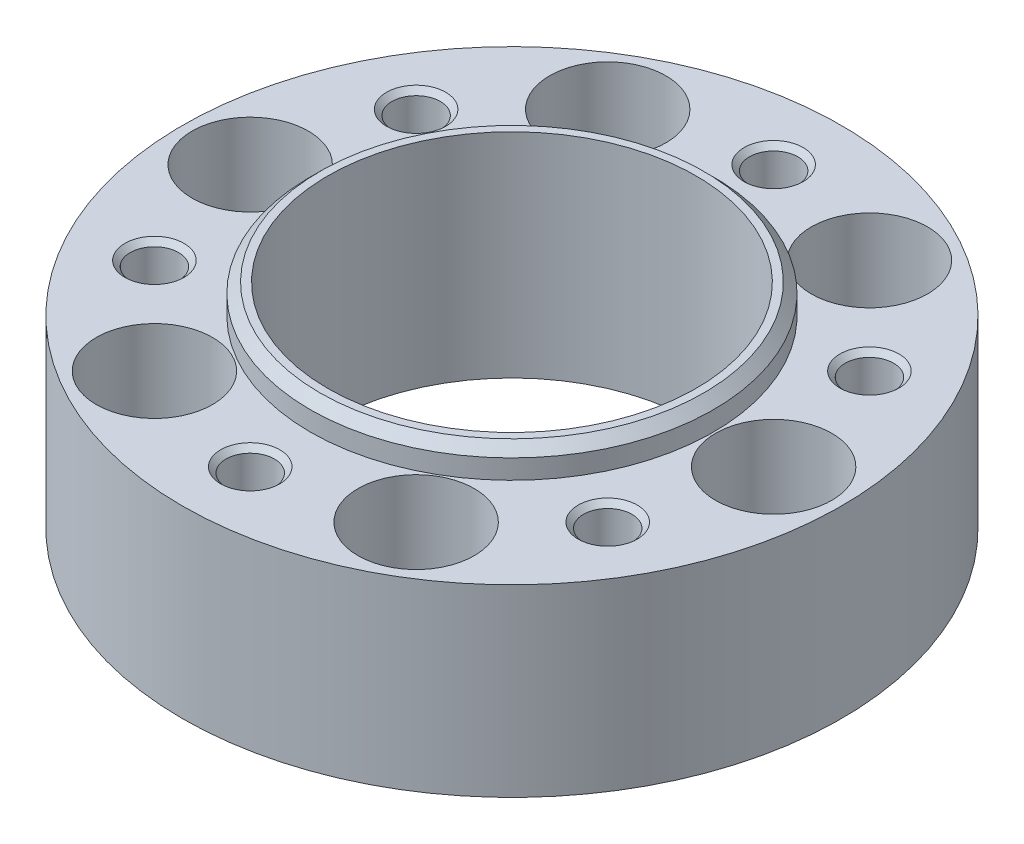
from build123d import *

# Parameters (mm, degrees)
SKETCH_1_R                   = 17
SKETCH_1_R_2                 = 1.55
SKETCH_1_R_3                 = 9.5
EXTRUDE_1_DEPTH              = 9.5
HOLE_WIZARD_M3_1_D           = 2.5
HOLE_WIZARD_M3_1_CSINK_D     = 3.05
HOLE_WIZARD_M3_1_CSINK_ANGLE = 90
SKETCH_7_R                   = 10.4
SKETCH_7_R_2                 = 9.5
EXTRUDE_2_DEPTH              = 1.5
SKETCH_5_R                   = 3
CUT_EXTRUDE_1_DEPTH          = 5.5
CHAMFER_1_SIZE               = 0.5


with BuildPart() as part:
    # 草图1 → 凸台-拉伸1 (new body)
    with BuildSketch(Plane(origin=(0, 0, 0), x_dir=(1, 0, 0), z_dir=(0, 1, 0))):
        with Locations(Location((0, 0, 0), (0, 0, 270))):
            Circle(SKETCH_1_R)
        with Locations(Location((13.5, 0, 0), (0, 0, 270))):
            Circle(SKETCH_1_R_2, mode=Mode.SUBTRACT)
        with Locations(Location((6.75, -11.691342951, 0), (0, 0, 270))):
            Circle(SKETCH_1_R_2, mode=Mode.SUBTRACT)
        with Locations(Location((-6.75, -11.691342951, 0), (0, 0, 270))):
            Circle(SKETCH_1_R_2, mode=Mode.SUBTRACT)
        with Locations(Location((-13.5, 0, 0), (0, 0, 270))):
            Circle(SKETCH_1_R_2, mode=Mode.SUBTRACT)
        with Locations(Location((-6.75, 11.691342951, 0), (0, 0, 270))):
            Circle(SKETCH_1_R_2, mode=Mode.SUBTRACT)
        with Locations(Location((6.75, 11.691342951, 0), (0, 0, 270))):
            Circle(SKETCH_1_R_2, mode=Mode.SUBTRACT)
        with Locations(Location((0, 0, 0), (0, 0, 270))):
            Circle(SKETCH_1_R_3, mode=Mode.SUBTRACT)
    extrude(amount=EXTRUDE_1_DEPTH)

    # M3 螺纹孔1 (through all)
    with Locations(Plane(origin=(0, 9.5, 0), x_dir=(1, 0, 0), z_dir=(0, 1, 0))):
        with Locations((11.691342951, 6.75), (11.691342951, -6.75), (0, -13.5), (-11.691342951, -6.75), (-11.691342951, 6.75), (0, 13.5), (0, 0)):
            CounterSinkHole(HOLE_WIZARD_M3_1_D / 2, HOLE_WIZARD_M3_1_CSINK_D / 2, counter_sink_angle=HOLE_WIZARD_M3_1_CSINK_ANGLE)

    # 草图7 → 凸台-拉伸2 (add)
    with BuildSketch(Plane(origin=(0, 9.5, 0), x_dir=(1, 0, 0), z_dir=(0, 1, 0))):
        with Locations(Location((0, 0, 0), (0, 0, 270))):
            Circle(SKETCH_7_R)
        with Locations(Location((0, 0, 0), (0, 0, 270))):
            Circle(SKETCH_7_R_2, mode=Mode.SUBTRACT)
    extrude(amount=EXTRUDE_2_DEPTH)

    # 草图5 → 切除-拉伸1 (cut)
    with BuildSketch(Plane(origin=(0, 9.5, 0), x_dir=(1, 0, 0), z_dir=(0, 1, 0))):
        with Locations(Location((13.5, 0, 0), (0, 0, 270))):
            Circle(SKETCH_5_R)
        with Locations(Location((6.75, -11.691342951, 0), (0, 0, 270))):
            Circle(SKETCH_5_R)
        with Locations(Location((-6.75, -11.691342951, 0), (0, 0, 270))):
            Circle(SKETCH_5_R)
        with Locations(Location((-13.5, 0, 0), (0, 0, 270))):
            Circle(SKETCH_5_R)
        with Locations(Location((-6.75, 11.691342951, 0), (0, 0, 270))):
            Circle(SKETCH_5_R)
        with Locations(Location((6.75, 11.691342951, 0), (0, 0, 270))):
            Circle(SKETCH_5_R)
    extrude(amount=-CUT_EXTRUDE_1_DEPTH, mode=Mode.SUBTRACT)

    # 倒角1
    chamfer_1_edges = [part.edges().sort_by_distance(p)[0] for p in [
        (0, 11, -10.4),
    ]]
    chamfer(chamfer_1_edges, length=CHAMFER_1_SIZE)


solid = part.part
